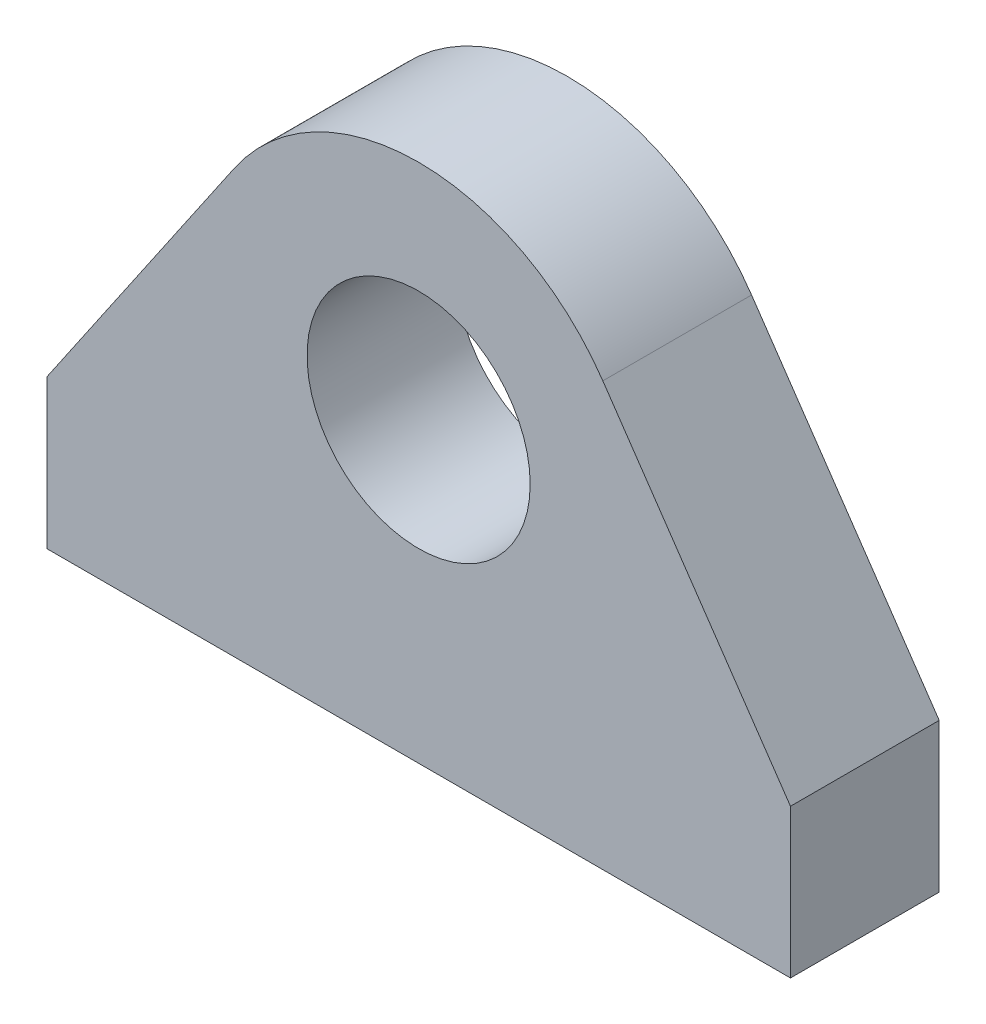
SolidWorks part; units mm, degrees
material "Q235-A"
ref_plane "前视基准面" through (0, 0, 0) normal (0, 0, 1) x (1, 0, 0)
ref_plane "上视基准面" through (0, 0, 0) normal (0, 1, 0) x (1, 0, 0)
ref_plane "右视基准面" through (0, 0, 0) normal (1, 0, 0) x (0, 0, -1)
sketch "草图1" plane through (0, 0, 0) normal (0, 0, 1) x (1, 0, 0)
  line L0 (0, 0) -> (0, -20) construction
  line L1 (25, -20) -> (-25, -20)
  line L2 (-25, -20) -> (-25, -10)
  line L3 (-25, -10) -> (-12.385, 8.4624)
  line L4 (25, -20) -> (25, -10)
  line L5 (25, -10) -> (12.385, 8.4624)
  circle A0 centre (0, 0) radius 7.5
  arc A1 (12.385, 8.4624) -> (-12.385, 8.4624) centre (0, 0) ccw
  dimension "D1" = 15
  dimension "D2" = 30
  dimension "D3" = 50
  dimension "D4" = 20
  dimension "D5" = 10
extrude "凸台-拉伸1" add sketch "草图1" along normal blind 10
